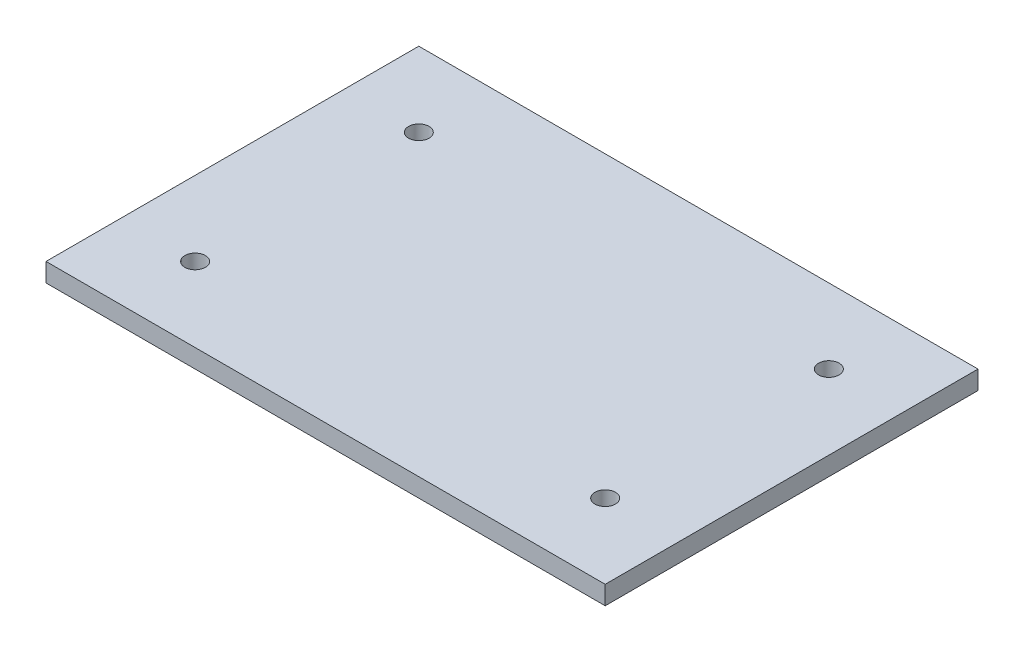
from build123d import *

# Parameters (mm, degrees)
SKETCH1_W           = 600
SKETCH1_H           = 400
BOSS_EXTRUDE1_DEPTH = 20
SKETCH2_R           = 11
CUT_EXTRUDE1_DEPTH  = 20


with BuildPart() as part:
    # Sketch1 → Boss-Extrude1 (new body)
    with BuildSketch(Plane(origin=(0, 0, 0), x_dir=(1, 0, 0), z_dir=(0, 1, 0))):
        Rectangle(SKETCH1_W, SKETCH1_H)
    extrude(amount=BOSS_EXTRUDE1_DEPTH)

    # Sketch2 → Cut-Extrude1 (cut)
    with BuildSketch(Plane(origin=(0, 20, 0), x_dir=(1, 0, 0), z_dir=(0, 1, 0))):
        with Locations(Location((-220, 120, 0), (0, 0, 270))):
            Circle(SKETCH2_R)
        with Locations(Location((220, 120, 0), (0, 0, 90))):
            Circle(SKETCH2_R)
        with Locations(Location((220, -120, 0), (0, 0, 270))):
            Circle(SKETCH2_R)
        with Locations(Location((-220, -120, 0), (0, 0, 90))):
            Circle(SKETCH2_R)
    extrude(amount=-CUT_EXTRUDE1_DEPTH, mode=Mode.SUBTRACT)


solid = part.part
